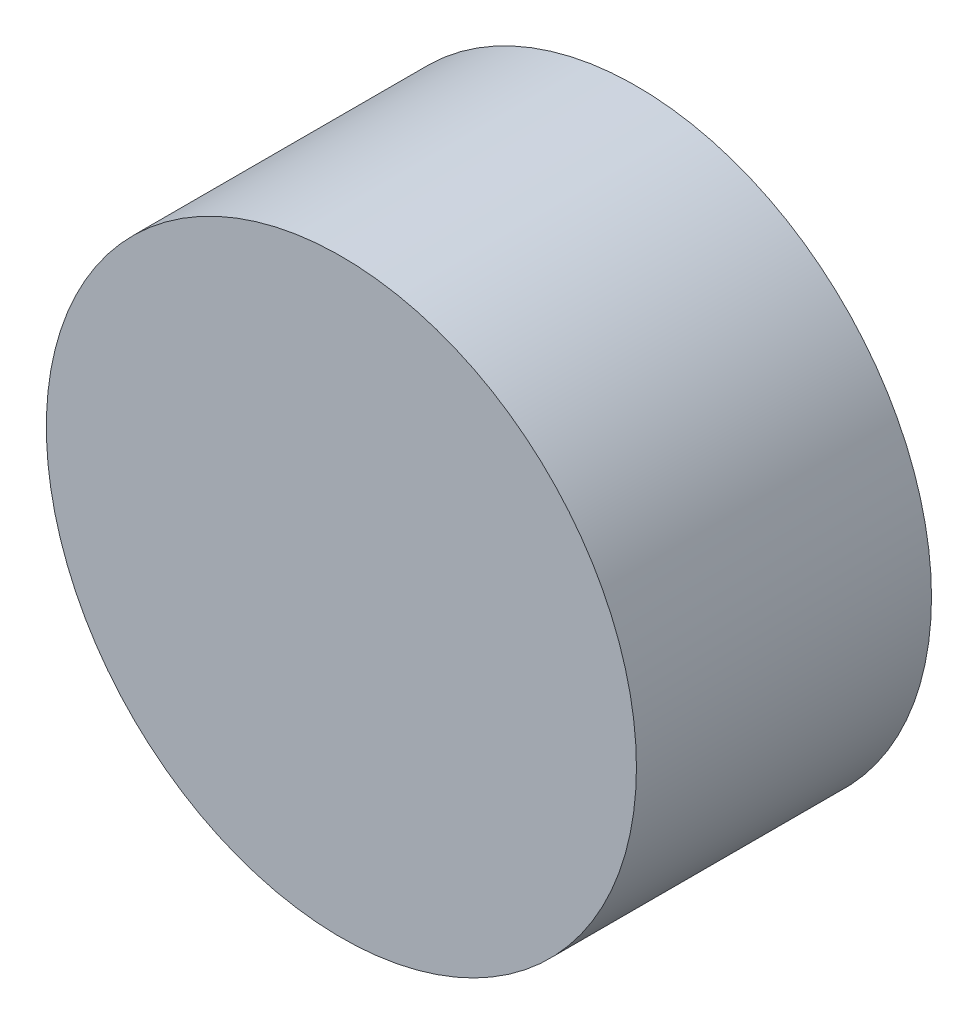
SolidWorks part; units mm, degrees
ref_plane "Front Plane" through (0, 0, 0) normal (0, 0, 1) x (1, 0, 0)
ref_plane "Top Plane" through (0, 0, 0) normal (0, 1, 0) x (1, 0, 0)
ref_plane "Right Plane" through (0, 0, 0) normal (1, 0, 0) x (0, 0, -1)
sketch "Sketch1" plane through (0, 0, 0) normal (0, 0, 1) x (1, 0, 0)
  circle A0 centre (0, 0) radius 6.35
extrude "Boss-Extrude1" add sketch "Sketch1" along normal blind 6.35
